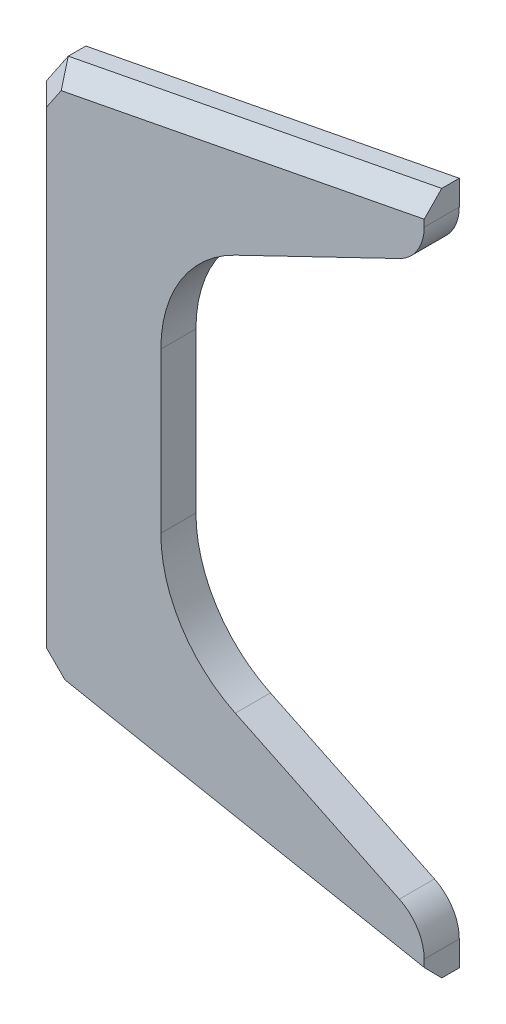
from build123d import *
from OCP.BRepFilletAPI import BRepFilletAPI_MakeChamfer

# Parameters (mm, degrees)
BOSS_EXTRUDE1_DEPTH = 16
CHAMFER1_SIZE       = 10
CHAMFER1_SIZE2      = 12.62624927
CHAMFER2_SIZE       = 8


with BuildPart() as part:
    # Sketch1 → Boss-Extrude1 (new body)
    with BuildSketch(Plane.XY):
        with BuildLine():
            Line((0, -121), (0, 121))
            Line((0, 121), (180, 155.8))
            Line((180, 155.8), (180, 144.470997586))
            ThreePointArc((180, 144.470997586), (176.937074168, 133.834479423), (168.686448136, 126.455847884))
            Line((168.686448136, 126.455847884), (93.940655591, 90.415323041))
            ThreePointArc((93.940655591, 90.415323041), (69.188777497, 68.279428426), (60, 36.369873936))
            Line((60, 36.369873936), (60, -36.269873936))
            ThreePointArc((60, -36.269873936), (69.188777497, -68.179428426), (93.940655591, -90.315323041))
            Line((93.940655591, -90.315323041), (168.686448136, -126.355847884))
            ThreePointArc((168.686448136, -126.355847884), (176.937074168, -133.734479423), (180, -144.370997586))
            Line((180, -144.370997586), (180, -155.8))
            Line((180, -155.8), (0, -121))
        make_face()
    extrude(amount=BOSS_EXTRUDE1_DEPTH)

    # Chamfer1: one chamfer whose edges measure the first distance from different faces: ONE call of the kernel's chamfer builder (chamfer() names one face for all edges)
    chamfer1_edges_1 = [part.edges().sort_by_distance(p)[0] for p in [
        (0, -121, 8),
    ]]
    chamfer1_side_1 = [part.faces().sort_by_distance(p)[0] for p in [
        (0, 0, 8),
    ]]
    chamfer1_edges_2 = [part.edges().sort_by_distance(p)[0] for p in [
        (0, 121, 8),
    ]]
    chamfer1_side_2 = [part.faces().sort_by_distance(p)[0] for p in [
        (90, 138.4, 8),
    ]]
    chamfer1 = BRepFilletAPI_MakeChamfer(part.part.solid().wrapped)
    for e in chamfer1_edges_1:
        chamfer1.Add(CHAMFER1_SIZE, CHAMFER1_SIZE2, e.wrapped, chamfer1_side_1[0].wrapped)  # the first distance lies on this face
    for e in chamfer1_edges_2:
        chamfer1.Add(CHAMFER1_SIZE, CHAMFER1_SIZE2, e.wrapped, chamfer1_side_2[0].wrapped)  # the first distance lies on this face
    add(Compound.cast(chamfer1.Shape()), mode=Mode.REPLACE)

    # Chamfer2
    chamfer2_edges = [part.edges().sort_by_distance(p)[0] for p in [
        (0, -1.313124635, 16),
        (96.198347107, -139.598347107, 16),
        (6.198347107, -117.198347107, 16),
        (4.909096102, 115.635967278, 16),
        (94.909096102, 139.349091913, 16),
    ]]
    chamfer(chamfer2_edges, length=CHAMFER2_SIZE)


solid = part.part
